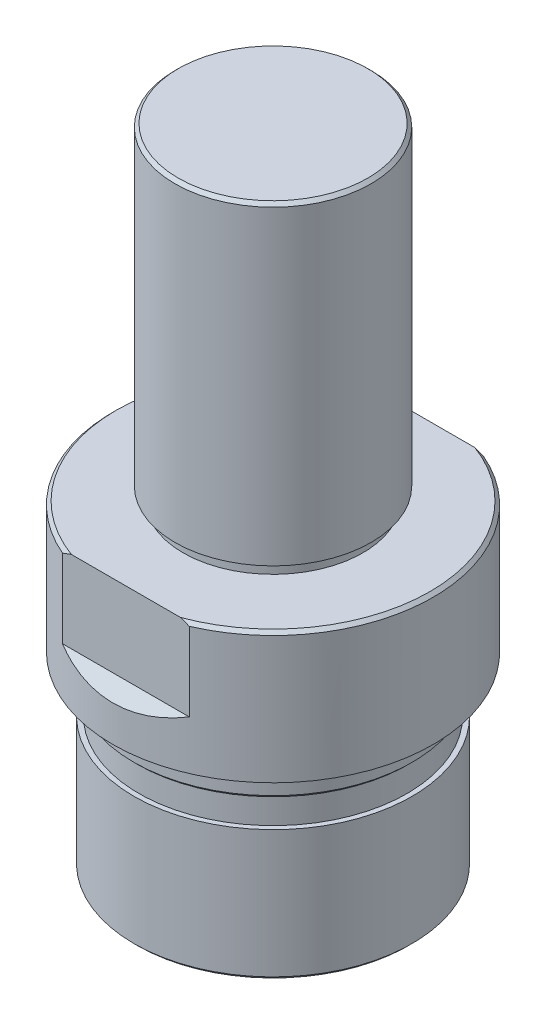
from build123d import *

# Parameters (mm, degrees)
SKETCH1_R           = 49
BOSS_EXTRUDE1_DEPTH = 40
SKETCH2_R           = 30
BOSS_EXTRUDE2_DEPTH = 100
SKETCH3_R           = 42.5
BOSS_EXTRUDE3_DEPTH = 9
SKETCH4_R           = 41
BOSS_EXTRUDE4_DEPTH = 8
SKETCH5_R           = 42.5
BOSS_EXTRUDE5_DEPTH = 40
CHAMFER1_SIZE       = 1
SKETCH6_W           = 154
SKETCH6_H           = 25
CUT_EXTRUDE1_DEPTH  = 25
CUT_EXTRUDE4_DEPTH  = 157.211395231
CUT_EXTRUDE5_DEPTH  = 157.211395231
SKETCH10_R          = 60.311534853
SKETCH10_R_2        = 27.5
CUT_EXTRUDE6_DEPTH  = 4
SKETCH13_R          = 25
CUT_EXTRUDE7_DEPTH  = 50


with BuildPart() as part:
    # Sketch1 → Boss-Extrude1 (new body)
    with BuildSketch(Plane(origin=(0, 0, 0), x_dir=(1, 0, 0), z_dir=(0, 1, 0))):
        with Locations(Location((0, 0, 0), (0, 0, 270))):
            Circle(SKETCH1_R)
    extrude(amount=BOSS_EXTRUDE1_DEPTH)

    # Sketch2 → Boss-Extrude2 (add)
    with BuildSketch(Plane(origin=(0, 40, 0), x_dir=(1, 0, 0), z_dir=(0, 1, 0))):
        with Locations(Location((0, 0, 0), (0, 0, 270))):
            Circle(SKETCH2_R)
    extrude(amount=BOSS_EXTRUDE2_DEPTH)

    # Sketch3 → Boss-Extrude3 (add)
    with BuildSketch(Plane.XZ):
        with Locations(Location((0, 0, 0), (0, 0, 90))):
            Circle(SKETCH3_R)
    extrude(amount=BOSS_EXTRUDE3_DEPTH)

    # Sketch4 → Boss-Extrude4 (add)
    with BuildSketch(Plane.XZ.offset(9)):
        with Locations(Location((0, 0, 0), (0, 0, 270))):
            Circle(SKETCH4_R)
    extrude(amount=BOSS_EXTRUDE4_DEPTH)

    # Sketch5 → Boss-Extrude5 (add)
    with BuildSketch(Plane.XZ.offset(17)):
        with Locations(Location((0, 0, 0), (0, 0, 90))):
            Circle(SKETCH5_R)
    extrude(amount=BOSS_EXTRUDE5_DEPTH)

    # Chamfer1
    chamfer1_edges = [part.edges().sort_by_distance(p)[0] for p in [
        (0, -9, -42.5),
        (0, -57, -42.5),
        (0, 40, -49),
        (0, 140, -30),
    ]]
    chamfer(chamfer1_edges, length=CHAMFER1_SIZE)

    # Sketch6 → Cut-Extrude1 (cut)
    with BuildSketch(Plane(origin=(0, 40, 0), x_dir=(1, 0, 0), z_dir=(0, 1, 0))):
        with Locations((0, 57.5)):
            Rectangle(SKETCH6_W, SKETCH6_H)
        with Locations((0, -57.5)):
            Rectangle(SKETCH6_W, SKETCH6_H)
    extrude(amount=-CUT_EXTRUDE1_DEPTH, mode=Mode.SUBTRACT)

    # Sketch 9_2 → Cut-Extrude4 (cut, through all)
    with BuildSketch(Plane(origin=(0, 0, 0), x_dir=(0, 0, -1), z_dir=(1, 0, 0))):
        Polygon((-45, 15), (-52.848399212, 15), (-52.983105111, 7.016894889), align=None)
        Polygon((45, 15), (54.94145121, 15), (54.048754667, 5.951245333), align=None)
    extrude(amount=-CUT_EXTRUDE4_DEPTH, mode=Mode.SUBTRACT)

    # Sketch 9_2 2 → Cut-Extrude5 (cut, through all)
    with BuildSketch(Plane(origin=(0, 0, 0), x_dir=(0, 0, -1), z_dir=(1, 0, 0))):
        Polygon((-45, 15), (-52.848399212, 15), (-52.983105111, 7.016894889), align=None)
        Polygon((45, 15), (54.94145121, 15), (54.048754667, 5.951245333), align=None)
    extrude(amount=CUT_EXTRUDE5_DEPTH, mode=Mode.SUBTRACT)

    # Sketch10 → Cut-Extrude6 (cut)
    with BuildSketch(Plane(origin=(0, 40, 0), x_dir=(1, 0, 0), z_dir=(0, 1, 0))):
        Circle(SKETCH10_R)
        with Locations(Location((0, 0, 0), (0, 0, 270))):
            Circle(SKETCH10_R_2, mode=Mode.SUBTRACT)
    extrude(amount=CUT_EXTRUDE6_DEPTH, mode=Mode.SUBTRACT)

    # Sketch13 → Cut-Extrude7 (cut)
    with BuildSketch(Plane.XZ.offset(57)):
        with Locations(Location((0, 0, 0), (0, 0, 270))):
            Circle(SKETCH13_R)
    extrude(amount=-CUT_EXTRUDE7_DEPTH, mode=Mode.SUBTRACT)


solid = part.part
